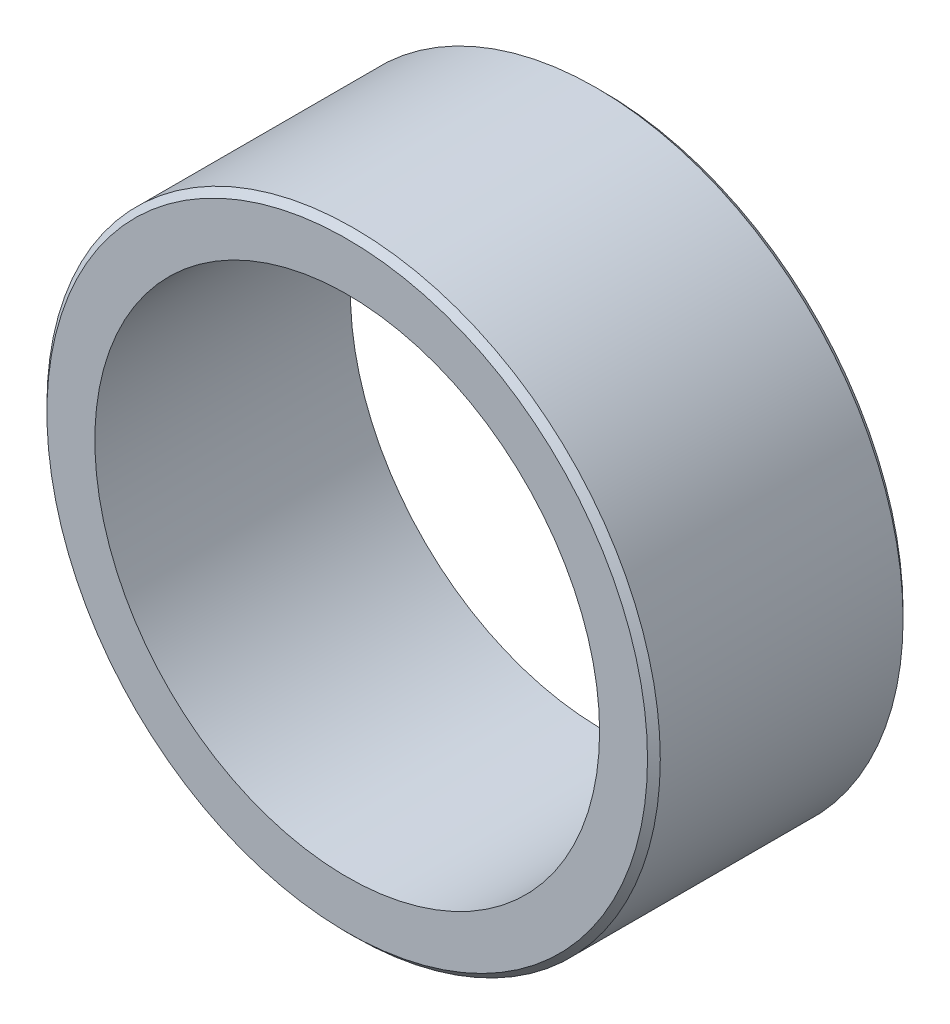
SolidWorks part; units mm, degrees
ref_plane "Front Plane" through (0, 0, 0) normal (0, 0, 1) x (1, 0, 0)
ref_plane "Top Plane" through (0, 0, 0) normal (0, 1, 0) x (1, 0, 0)
ref_plane "Right Plane" through (0, 0, 0) normal (1, 0, 0) x (0, 0, -1)
sketch "Sketch1" plane through (0, 0, 0) normal (0, 0, 1) x (1, 0, 0)
  circle A0 centre (0, 0) radius 24
  circle A1 centre (0, 0) radius 19.75
  dimension "D1" = 48
  dimension "D2" = 39.5
extrude "Boss-Extrude1" add sketch "Sketch1" along normal mid plane 20
chamfer "Chamfer1" distance 0.5 angle 45 2 edges at (24, 0, -10) (24, 0, 10)
